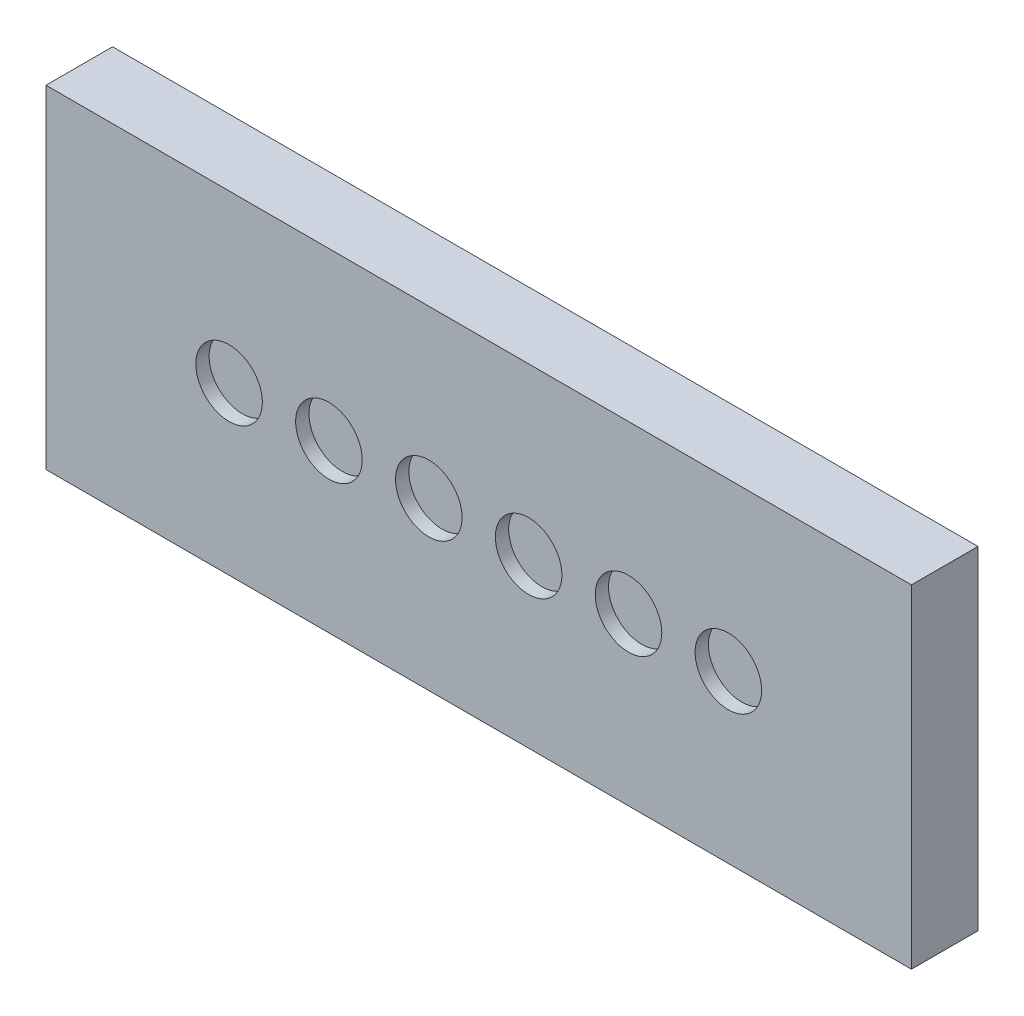
from build123d import *

# Parameters (mm, degrees)
SKETCH1_W           = 130
SKETCH1_H           = 50
BOSS_EXTRUDE1_DEPTH = 10
SKETCH2_R           = 5
CUT_EXTRUDE1_DEPTH  = 2


with BuildPart() as part:
    # Sketch1 → Boss-Extrude1 (new body)
    with BuildSketch(Plane.XY):
        Rectangle(SKETCH1_W, SKETCH1_H)
    extrude(amount=BOSS_EXTRUDE1_DEPTH)

    # Sketch2 → Cut-Extrude1 (cut)
    with BuildSketch(Plane.XY.offset(10)):
        with Locations((-37.5, 0)):
            Circle(SKETCH2_R)
        with Locations((-22.5, 0)):
            Circle(SKETCH2_R)
        with Locations((-7.5, 0)):
            Circle(SKETCH2_R)
        with Locations((7.5, 0)):
            Circle(SKETCH2_R)
        with Locations((22.5, 0)):
            Circle(SKETCH2_R)
        with Locations((37.5, 0)):
            Circle(SKETCH2_R)
    extrude(amount=-CUT_EXTRUDE1_DEPTH, mode=Mode.SUBTRACT)


solid = part.part
